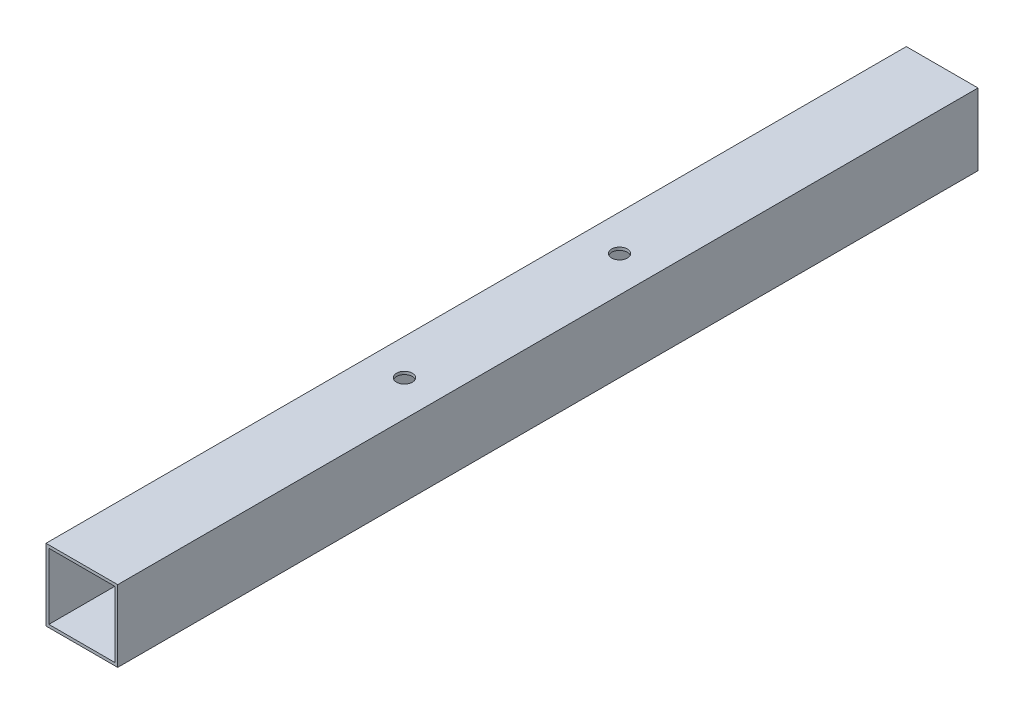
from build123d import *

# Parameters (mm, degrees)
SKETCH1_W           = 50
SKETCH1_H           = 50
SKETCH1_W_2         = 46
SKETCH1_H_2         = 46
BOSS_EXTRUDE1_DEPTH = 600
SKETCH2_R           = 5.5
CUT_EXTRUDE1_DEPTH  = 50


with BuildPart() as part:
    # Sketch1 → Boss-Extrude1 (new body)
    with BuildSketch(Plane.XY):
        Rectangle(SKETCH1_W, SKETCH1_H)
        Rectangle(SKETCH1_W_2, SKETCH1_H_2, mode=Mode.SUBTRACT)
    extrude(amount=BOSS_EXTRUDE1_DEPTH)

    # Sketch2 → Cut-Extrude1 (cut)
    with BuildSketch(Plane(origin=(0, 25, 0), x_dir=(1, 0, 0), z_dir=(0, 1, 0))):
        with Locations(Location((0, -225, 0), (0, 0, 270))):
            Circle(SKETCH2_R)
        with Locations(Location((0, -375, 0), (0, 0, 270))):
            Circle(SKETCH2_R)
    extrude(amount=-CUT_EXTRUDE1_DEPTH, mode=Mode.SUBTRACT)


solid = part.part
